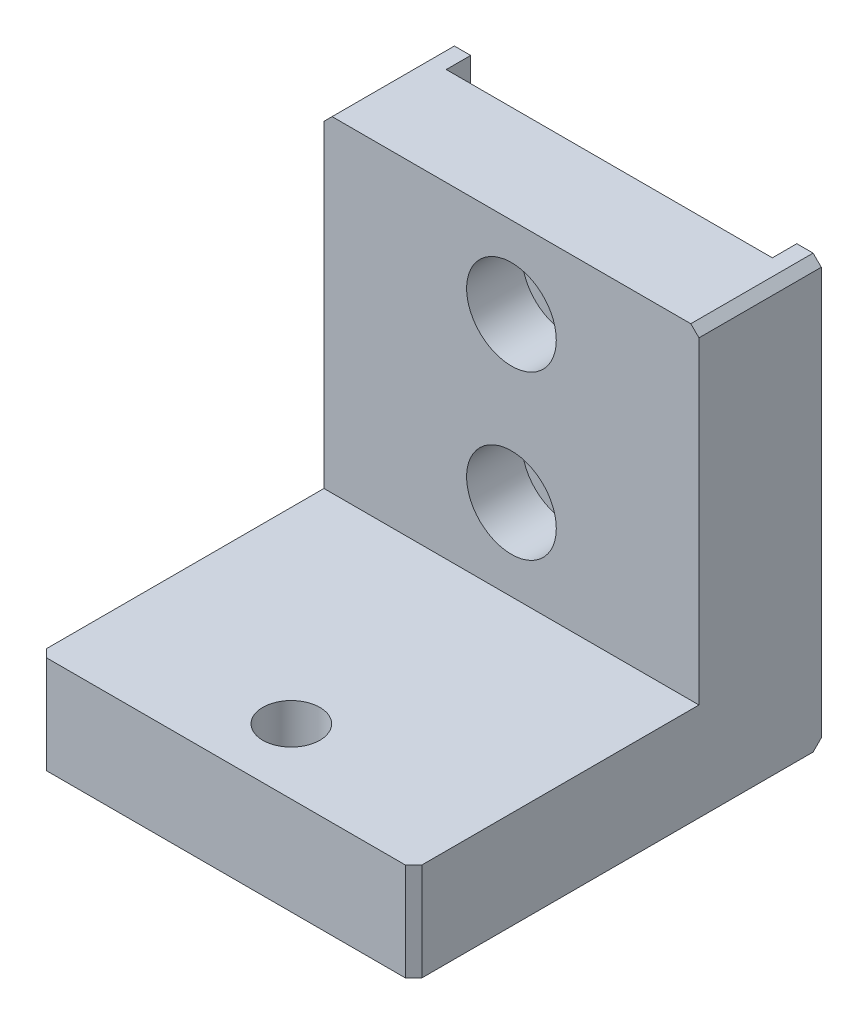
SolidWorks part; units mm, degrees
material "A6061"
ref_plane "前基準面" through (0, 0, 0) normal (0, 0, 1) x (1, 0, 0)
ref_plane "上基準面" through (0, 0, 0) normal (0, 1, 0) x (1, 0, 0)
ref_plane "右基準面" through (0, 0, 0) normal (1, 0, 0) x (0, 0, -1)
sketch "草图1" plane through (0, 0, 0) normal (0, 1, 0) x (1, 0, 0)
  line L1 (-23, -25) -> (23, -25)
  line L2 (-23, -25) -> (-23, 25)
  line L3 (-23, 25) -> (23, 25)
  line L4 (23, -25) -> (23, 25)
  line L5 (-23, -25) -> (23, 25) construction
  line L6 (-23, 25) -> (23, -25) construction
  point P0 (0, 0)
  dimension "D1" = 46
  dimension "D2" = 50
extrude "凸台-拉伸1" add sketch "草图1" along normal mid plane 12
sketch "草图2" plane through (0, 6, 0) normal (0, 1, 0) x (1, 0, 0)
  line L0 (23, -25) -> (23, 25) construction
  line L1 (23, 25) -> (-23, 25)
  line L2 (23, 25) -> (23, 10)
  line L3 (23, 10) -> (-23, 10)
  line L4 (-23, 25) -> (-23, 10)
  line L5 (-23, 25) -> (-23, -25) construction
  line L6 (23, 25) -> (-23, 25) construction
  dimension "D1" = 15
extrude "凸台-拉伸2" add sketch "草图2" along normal blind 40
sketch "草图3" plane through (0, 0, -25) normal (0, 0, -1) x (-1, 0, 0)
  line L0 (-23, 46) -> (23, 46) construction
  line L1 (-20, 46) -> (20, 46)
  line L2 (-20, 46) -> (-20, -6)
  line L3 (-20, -6) -> (20, -6)
  line L4 (20, 46) -> (20, -6)
  line L5 (-23, -6) -> (23, -6) construction
  line L6 (0, 46) -> (0, 0) construction
  dimension "D1" = 40
extrude "切除-拉伸1" cut sketch "草图3" against normal blind 3
chamfer "倒角1" distance 1 angle 45 5 edges at (23, 0, 25) (-23, 0, 25) (-23, 46, -17.5) (23, 46, -17.5) (-21.5, -6, -25)
hole_wizard "打孔尺寸(%根据)内六角圆柱头螺钉的类型1" positions "草图4" profile "草图5" counterbore size "M6" standard "GB" end condition through all
sketch "草图4" plane through (0, 0, -10) normal (0, 0, 1) x (1, 0, 0)
  line L0 (-22, 46) -> (22, 46) construction
  point P0 (0, 16)
  point P2 (0, 36)
  dimension "D1" = 20
  dimension "D2" = 10
sketch "草图5" plane through (0, 16, -10) normal (1, 0, 0) x (0, -1, 0)
  line L0 (0, 0) -> (0, 15)
  line L1 (0, 15) -> (3.3, 15)
  line L3 (3.3, 15) -> (3.3, 6.8)
  line L4 (3.3, 6.8) -> (5.5, 6.8)
  line L5 (5.5, 6.8) -> (5.5, 0)
  line L7 (5.5, 0) -> (0, 0)
  line L11 (0, -6.35) -> (0, 107.95) construction
  dimension "通孔孔直径" = 6.6
  dimension "通孔孔深度" = 15
  dimension "柱形沉头孔直径" = 11
  dimension "柱形沉头孔深度" = 6.8
hole_wizard "M8x1.0 螺纹孔1" positions "草图6" profile "草图7" tap size "M8x1.0" standard "GB" end condition through all
sketch "草图6" plane through (0, 6, 0) normal (0, 1, 0) x (1, 0, 0)
  line L0 (-22, -25) -> (22, -25) construction
  point P0 (0, -17)
  dimension "D1" = 8
sketch "草图7" plane through (0, 6, 17) normal (1, 0, 0) x (0, 0, 1)
  line L0 (0, 0) -> (0, 12)
  line L1 (0, 12) -> (3.5, 12)
  line L2 (3.5, 12) -> (3.5, 0)
  line L5 (3.5, 0) -> (0, 0)
  line L11 (0, -6.35) -> (0, 107.95) construction
  dimension "通孔螺纹孔钻头直径" = 7
  dimension "通孔螺纹孔钻头深度" = 12
cosmetic thread "孔螺蚊线1" parameters "D2"=8
